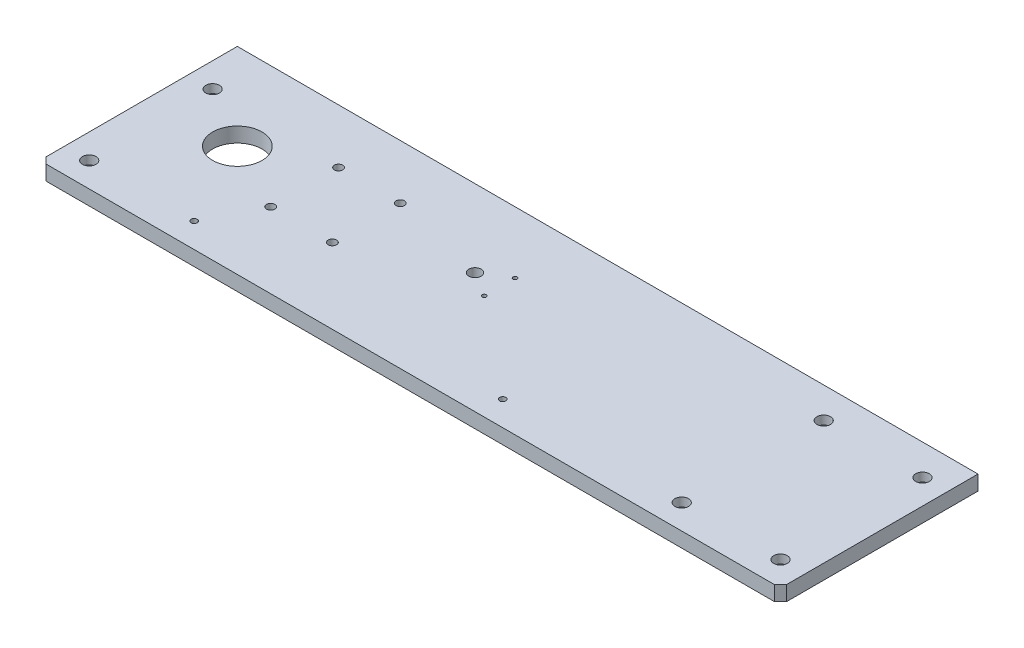
from build123d import *

# Parameters (mm, degrees)
SKETCH1_W                                         = 600
SKETCH1_H                                         = 160
EXTRUDE1_DEPTH                                    = 6
M6_SOCKET_HEAD_CAP_SCREW_COUNTERBORE1_D           = 6.6
M6_SOCKET_HEAD_CAP_SCREW_COUNTERBORE1_CBORE_D     = 11
M6_SOCKET_HEAD_CAP_SCREW_COUNTERBORE1_CBORE_DEPTH = 7
M4_TAPPED_HOLE1_D                                 = 3.3
M4_TAPPED_HOLE1_DEPTH                             = 10.1
M4_TAPPED_HOLE1_TIP                               = 0.991420021
M8_TAPPED_HOLE1_D                                 = 6.8
M6_TAPPED_HOLE2_D                                 = 5
SKETCH10_R                                        = 20
CUT_EXTRUDE1_DEPTH                                = 311.715303775
M4_TAPPED_HOLE2_D                                 = 3.3
M4_TAPPED_HOLE2_DEPTH                             = 12
M4_TAPPED_HOLE2_TIP                               = 0.991420021
CHAMFER1_SIZE                                     = 5
SKETCH13_R                                        = 5
CUT_EXTRUDE2_DEPTH                                = 311.715303775


with BuildPart() as part:
    # Sketch1 → Extrude1 (new, symmetric)
    with BuildSketch(Plane(origin=(0, 0, 0), x_dir=(1, 0, 0), z_dir=(0, 1, 0))):
        Rectangle(SKETCH1_W, SKETCH1_H)
    extrude(amount=EXTRUDE1_DEPTH, both=True)

    # M6 Socket Head Cap Screw Counterbore1 (through all)
    with Locations(Plane(origin=(-280, 6, 60), x_dir=(0, 0, 1), z_dir=(0, 1, 0))):
        with Locations((0, 0), (-100, 0), (0, 480), (-115, 480), (-115, 560), (0, 560)):
            CounterBoreHole(M6_SOCKET_HEAD_CAP_SCREW_COUNTERBORE1_D / 2, M6_SOCKET_HEAD_CAP_SCREW_COUNTERBORE1_CBORE_D / 2, M6_SOCKET_HEAD_CAP_SCREW_COUNTERBORE1_CBORE_DEPTH)

    # M4 Tapped Hole1
    with Locations(Plane(origin=(270, 0, -80), x_dir=(-1, 0, 0), z_dir=(0, 0, -1))):
        with Locations((0, 0), (250, 0), (500, 0)):
            Hole(M4_TAPPED_HOLE1_D / 2, depth=M4_TAPPED_HOLE1_DEPTH)
            with Locations((0, 0, -(M4_TAPPED_HOLE1_DEPTH + M4_TAPPED_HOLE1_TIP / 2))):  # 118° drill point
                Cone(0, M4_TAPPED_HOLE1_D / 2, M4_TAPPED_HOLE1_TIP, mode=Mode.SUBTRACT)

    # M8 Tapped Hole1 (through all)
    with Locations(Plane(origin=(-174, 6, 19), x_dir=(0, 0, 1), z_dir=(0, 1, 0))):
        with Locations((0, 0), (0, 50), (-55, 50), (-55, 0)):
            Hole(M8_TAPPED_HOLE1_D / 2)

    # M6 Tapped Hole2 (through all)
    with Locations(Plane(origin=(55, 6, 60), x_dir=(0, 0, 1), z_dir=(0, 1, 0))):
        with Locations((0, 0), (0, -250)):
            Hole(M6_TAPPED_HOLE2_D / 2)

    # Sketch10 → Cut-Extrude1 (cut, through all)
    with BuildSketch(Plane(origin=(0, 6, 0), x_dir=(1, 0, 0), z_dir=(0, 1, 0))):
        with Locations(Location((-230, 10, 0), (0, 0, 270))):
            Circle(SKETCH10_R)
    extrude(amount=-CUT_EXTRUDE1_DEPTH, mode=Mode.SUBTRACT)

    # M4 Tapped Hole2
    with Locations(Plane(origin=(-25, 6, -5), x_dir=(0, 0, 1), z_dir=(0, 1, 0))):
        with Locations((0, 0), (-25, 0)):
            Hole(M4_TAPPED_HOLE2_D / 2, depth=M4_TAPPED_HOLE2_DEPTH)
            with Locations((0, 0, -(M4_TAPPED_HOLE2_DEPTH + M4_TAPPED_HOLE2_TIP / 2))):  # 118° drill point
                Cone(0, M4_TAPPED_HOLE2_D / 2, M4_TAPPED_HOLE2_TIP, mode=Mode.SUBTRACT)

    # Chamfer1
    chamfer1_edges = [part.edges().sort_by_distance(p)[0] for p in [
        (300, 0, 80),
        (-300, 0, 80),
    ]]
    chamfer(chamfer1_edges, length=CHAMFER1_SIZE)

    # Sketch13 → Cut-Extrude2 (cut, through all)
    with BuildSketch(Plane(origin=(0, 6, 0), x_dir=(1, 0, 0), z_dir=(0, 1, 0))):
        with Locations(Location((-45, 17.5, 0), (0, 0, 270))):
            Circle(SKETCH13_R)
    extrude(amount=-CUT_EXTRUDE2_DEPTH, mode=Mode.SUBTRACT)


solid = part.part
